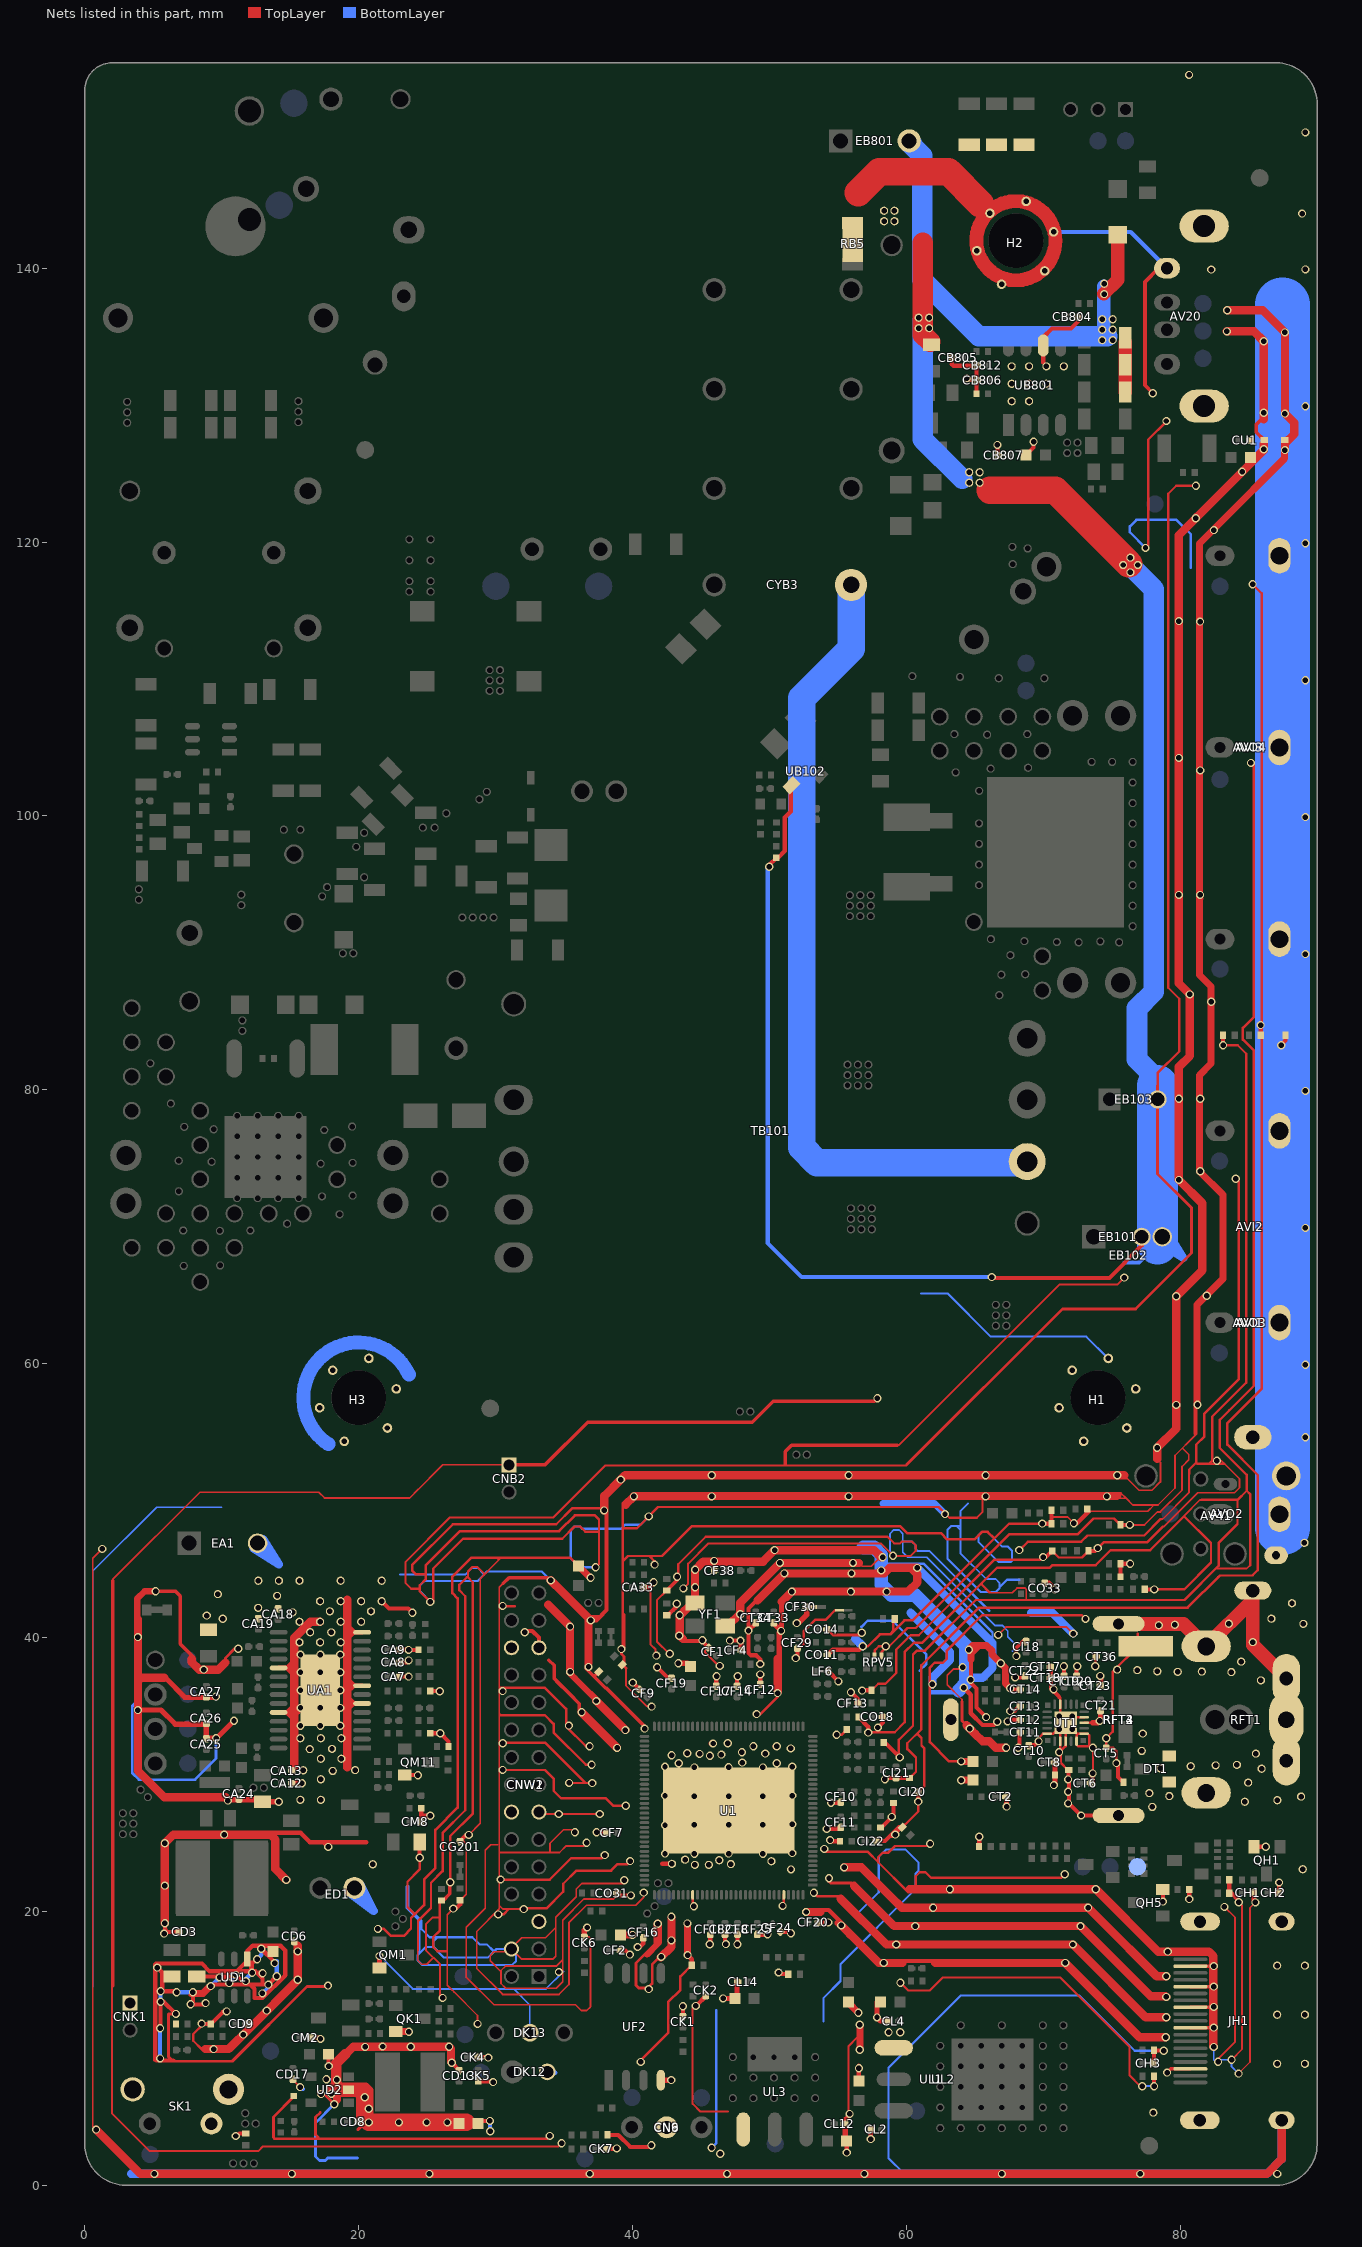
[diagram p0: the nets of this part, all layers, seen from the top]
# Altium PCB MISC116569.PcbDoc (part 9 of 15)
Units mm, origin at the board's own origin, x right, y up, seen from the top; angles counter-clockwise.
Board outline 90 x 155 mm, 2 copper layers (TopLayer, BottomLayer), stack 1.571 mm thick; 527 components, 277 nets, 2450 pads, 649 vias.

## Via types
v1: diameter 0.6, hole 0.4, TopLayer to BottomLayer, tented both sides, 649 vias

## Nets (pads, with @x,y where several pads share a name; then routed paths per layer and width w, separated by ;. In a path a pad name is that pad's centre, name@x,y a point inside that pad or via, vN(x,y) a via of type N, cw(c..) or ccw(c..) an arc to the next point about the centre after c; other vN are vias at no path point) (continued)
GND: (continued)
  TopLayer w0.3: v1(32.131,40.386) 32.233,40.488 32.677,40.488 33.164,40.001 CNW2.25@33.164,39.251 ; CF2.1@39.138,17.147 39.495,17.147 39.802,16.84 v1(39.816,16.84) ; v1(49.987,96.291) 49.854,96.291 RB134.1@50.503,96.94 v1@50.013,96.45 ; RB134.1@50.627,96.939 51.119,97.431 51.119,99.009 ; UB102.A@51.556,102.274 51.556,100.317 ; 63.32,132.992 CB805.2@63.32,133.477 ; v1(66.23,66.319) 66.285,66.265 74.837,66.265 77.187,68.615 EB101.2@77.187,69.266 ; 69.998,133.117 UB801.6@69.998,134.358 69.998,134.958 70.637,135.598 72.022,135.598 72.523,136.099 CB804.1@72.523,136.398 ; 51.119,99.009 51.119,99.88 51.556,100.317 ; 51.119,99.009 51.119,99.888 51.341,100.11 51.349,100.11 51.556,100.317
  TopLayer w0.305: 5.151,9.139 5.151,9.335 ; v1(5.299,15.89) 5.658,15.531 5.658,14.16 v1(5.532,14.16) 6.637,14.16 v1(6.701,14.097) ; v1@5.494,9.144 v1(5.494,9.258) ; v1(5.498,11.468) 5.536,11.506 v1(5.536,13.399) 5.763,13.399 v1(6.651,12.51) ; v1(5.791,18.377) 5.791,18.466 5.829,18.504 CD3.1@6.851,18.504 6.053,18.504 5.85,18.707 v1(5.85,19.139) ; 6.459,9.106 5.228,9.106 5.151,9.182 5.151,9.335 ; v1@7.742,13.881 8.664,13.881 9.438,14.655 12.987,14.655 ; CD1.2@8.174,15.241 10.717,15.241 UD1.1@11.855,16.38 ; v1(8.526,11.805) 8.558,11.773 RD6.1@9.204,11.773 10.118,12.687 v1(10.358,12.687) ; v1(8.822,13.297) 8.733,13.208 v1(7.729,13.208) 7.895,13.373 v1(7.895,14.097) 8.553,14.097 8.998,14.541 v1(9.203,14.541) ; v1(9.838,15.176) 10.128,15.176 v1(10.549,14.757) v1(10.549,14.757) ; v1(11.019,3.594) 11.07,3.543 11.291,3.765 DK1.A@11.562,3.765 ; v1(11.031,15.354) 11.476,14.91 v1(11.755,14.91) ; v1(11.572,11.003) 11.859,11.291 CD9.1@11.859,11.786 ; UD1.1@11.867,16.525 11.867,17.092 12.26,17.485 14.305,17.485 14.638,17.152 14.638,15.327 12.976,13.665 12.396,13.665 12.396,14.344 12.086,14.655 ; 12.149,16.243 12.149,15.587 v1(12.214,15.523) ; v1(12.581,16.497) 12.532,16.497 12.214,16.179 v1(12.214,15.523) ; v1(12.886,17.272) 13.864,16.294 v1(13.864,16.218) ; v1@12.917,13.951 v1(12.975,14.008) ; v1(12.979,15.481) 12.938,15.523 v1(12.214,15.523) ; v1@13.215,14.655 12.987,14.655 ; v1(13.295,12.756) 13.398,12.756 15.548,14.906 v1(15.548,15.009) ; v1(13.413,14.649) v1(14.022,15.259) ; CD6.1@15.299,17.749 15.553,17.495 v1(15.553,17.069) ; CM2.1@16.536,10.782 17.114,10.782 v1(17.214,10.682) ; CD16.1@17.808,9.563 17.808,8.704 v1(17.813,8.7) ; v1(20.445,6.426) 20.445,5.877 v1(20.745,5.577) ; v1(20.471,10.103) 20.133,10.103 20.107,10.13 v1(21.75,10.13) ; v1(20.745,4.585) v1(22.944,4.585) ; pad.VIA5@21.68,42.649 22.216,42.113 23.622,42.113 v1(23.927,41.808) ; CA7.1@22.964,37.145 23.64,37.145 v1(23.643,37.148) ; CA8.1@22.964,38.177 23.491,38.177 v1(23.643,38.329) ; CA9.1@22.964,39.107 23.626,39.107 v1(23.643,39.091) RA11.1@24.363,39.091 ; QM11.E@23.363,29.947 v1(24.328,29.947) ; v1(23.808,10.109) 24.76,10.109 ; v1(24.455,23.914) CM7.2@24.455,25.07 ; CM8.1@24.575,26.53 24.575,26.987 ; RM15.2@24.575,27.533 24.575,26.987 ; v1(24.963,4.585) 25.725,4.585 ; RA1.2@25.229,33.011 v1(25.958,33.011) 26.569,32.4 RM12.2@26.569,32.029 ; RA9.1@25.229,36.087 25.91,36.087 v1(25.916,36.081) ; v1(25.23,26.987) 24.575,26.987 ; v1(26.487,4.585) 27.851,4.585 ; v1(26.805,8.943) 26.811,8.943 CD13.1@27.338,8.416 ; v1(26.909,20.203) 26.91,20.201 27.116,20.201 27.414,20.499 RF13.2@27.414,20.812 ; CD15.1@27.345,4.49 CD15.1@27.413,4.559 ; CG201.2@27.414,25.144 27.85,25.58 v1(28.037,25.58) ; CD14.1@28.729,4.49 28.937,4.699 v1(29.591,4.699) ; CK5.2@28.735,7.566 29.7,7.566 v1@29.737,7.529 ; CK4.2@28.766,9.362 29.434,9.362 v1(29.472,9.324) ; v1(37.38,25.774) 37.395,25.758 CF7.1@38.057,25.758 ; CK7.2@38.156,2.657 38.819,2.657 v1(38.844,2.682) ; DK3.A@38.164,3.673 38.961,3.673 39.841,2.792 40.927,2.792 ; CO31.1@38.907,21.338 39.085,21.161 v1(39.886,21.161) ; v1(40.013,36.705) CF9.1@40.5,36.218 ; v1(40.372,17.397) 40.542,17.397 40.787,17.643 CF16.1@40.787,18.031 ; CA33.1@40.835,43.665 41.245,43.665 41.537,43.957 v1(41.537,44.033) ; v1(41.384,2.911) 41.266,2.792 40.927,2.792 ; v1@41.388,2.792 40.927,2.792 ; v1(41.796,37.833) 42.56,37.069 CF19.2@42.85,37.069 ; DI10.A@42.489,41.627 42.598,41.627 42.934,41.963 ; 43.124,42.154 42.934,41.963 ; v1(43.226,42.459) 43.188,42.459 43.162,42.484 43.162,42.192 42.934,41.963 ; v1@43.454,40.123 43.841,39.736 ; CK1.1@43.683,12.361 v1(43.683,13.071) ; 43.689,39.888 43.841,39.736 ; v1(44.023,16.808) 44.33,16.501 D102.A@44.33,16.081 ; v1(44.623,13.096) 44.597,13.122 44.667,13.122 CK2.2@45.347,13.801 ; v1@45.171,39.736 44.526,39.736 ; CF1.1@45.545,39.265 45.11,39.7 v1(45.11,39.802) 45.045,39.736 44.526,39.736 ; v1(45.639,17.605) 45.683,17.648 CF18.2@45.683,18.283 ; CF38.1@45.951,44.884 45.951,45.587 v1(45.956,45.593) ; CF17.1@46.114,36.491 46.114,37.147 v1(46.136,37.169) ; CF21.2@46.749,18.283 46.749,17.681 v1(46.824,17.605) ; v1(47.112,39.778) 47.113,39.779 v1(47.887,39.779) 47.887,39.141 CF4.1@47.96,39.068 v1@47.96,39.769 ; CF14.1@47.638,36.491 47.638,37.124 v1(47.683,37.169) ; v1(47.658,17.605) 47.666,17.613 CF8.1@47.666,18.283 ; CF12.1@49.335,36.622 v1(49.335,37.302) ; v1@49.335,38.292 v1(49.335,38.064) 49.335,38.398 49.031,38.701 48.647,38.701 48.471,38.877 48.471,40.5 CT34.2@49.002,41.031 48.474,40.503 v1(48.471,40.503) 48.471,42.118 49.452,43.099 ; 49.474,18.283 CF25.2@49.112,18.283 49.814,18.283 v1(49.863,18.332) ; v1(50.668,15.535) 50.782,15.42 D101.A@51.373,15.42 ; CF24.2@50.825,18.491 51.48,18.491 v1(51.567,18.404) ; v1(51.918,38.494) v1@52.04,38.616 ; v1@52.04,38.712 CF29.2@52.04,39.18 ; 53.157,19.953 53.31,20.105 54.334,20.105 55.878,18.56 ; CF20.1@53.612,19.192 v1(54.3,19.192) ; v1(54.178,26.022) 54.185,26.029 CF11.2@55.207,26.029 ; CO11.1@54.26,38.735 54.627,39.102 55.156,39.102 ; LF6.1@54.331,37.502 v1(55.042,36.792) v1@55.019,36.792 ; v1(54.432,25.209) 54.521,25.121 RV5.1@55.157,25.121 ; v1(54.496,27.927) 54.499,27.93 CF10.1@55.207,27.93 ; 54.772,39.102 55.156,39.102 ; v1(55.642,2.382) CL11.1@55.642,3.241 ; v1(55.956,36.005) 56.495,35.465 CF13.1@56.495,35.204 ; RO18.1@56.496,34.194 57.213,33.476 v1(57.213,33.058) ; v1(56.769,36.119) 56.794,36.144 DV7.A@57.462,36.144 ; v1(56.815,39.36) 56.557,39.102 55.156,39.102 ; CL2.1@57.393,4.079 57.393,3.374 v1(57.399,3.368) ; CI22.2@57.812,25.133 58.445,25.133 58.839,25.527 ; v1(57.925,33.426) 58.293,33.794 CO18.1@58.293,34.194 ; RF16.2@58.102,26.112 58.177,26.112 v1@58.928,26.863 ; RI18.1@58.346,32.334 58.43,32.334 v1@59.459,31.306 ; v1(58.433,29.642) 58.522,29.731 RV1.1@60.236,29.731 ; v1(58.928,26.899) v1@58.928,26.863 ; RV3.1@59.055,27.909 59.055,26.99 v1@58.928,26.863 ; v1(59.182,25.603) 59.106,25.527 58.839,25.527 ; 59.266,16.385 61.958,16.385 62.111,16.233 ; DV9.A@59.686,26.153 59.466,26.153 58.839,25.527 ; v1(60.871,28.016) CI20.2@60.871,28.727 ; 63.32,132.992 63.44,132.871 65.068,132.871 CB812.2@65.115,132.918 RB803.1@65.115,130.835 ; v1(64.186,36.335) 64.702,35.819 64.702,35.369 ; v1(64.414,131.953) 64.541,131.826 CB806.2@65.115,131.826 ; v1(64.691,36.909) 64.714,36.932 64.714,37.478 ; 64.702,35.608 64.702,35.369 ; 64.702,35.641 64.702,35.369 ; 64.714,38.832 64.714,37.478 ; 65.121,36.045 65.121,35.827 ; RH82.2@65.317,24.74 65.317,25.45 v1(65.316,25.451) ; v1(65.819,34.191) 65.121,34.889 65.121,35.827 ; v1(66.632,33.848) 66.399,33.615 65.556,33.615 64.702,34.47 64.702,35.369 ; CB807.1@66.652,126.34 v1(66.652,127.095) ; v1(67.394,33.873) 67.508,33.988 CT12.1@68.258,33.988 ; v1(67.581,34.631) 67.911,34.631 CT13.2@68.258,34.978 ; v1(67.584,36.299) 67.673,36.21 CT14.1@68.265,36.21 ; v1(67.94,37.086) 68.61,37.086 CT22.2@68.664,37.14 ; v1(68.169,31.956) 68.258,32.045 CT11.1@68.258,33.079 ; CB801.2@68.75,126.362 69.286,126.899 v1(69.286,127.33) ; CT10.1@68.943,32.139 69.368,32.139 v1(69.655,32.426) ; v1(69.931,48.317) 69.935,48.313 DI1.A@70.608,48.313 DA32.A@70.608,49.291 ; v1(69.98,45.876) 70.209,45.876 RO4.1@70.652,46.319 ; CO33.1@70.104,44.011 70.416,44.011 70.841,43.586 v1(70.841,43.523) ; CT17.2@70.558,37.848 70.558,36.69 ; v1(70.754,36.219) 70.738,36.219 70.558,36.399 70.558,36.69 ; 71.138,35.679 70.558,36.258 70.558,36.69 ; v1(71.505,37.897) 71.522,37.88 CT19.1@71.522,37.219 ; v1@71.852,29.784 LT4.1@71.852,30.324 ; v1@71.877,29.632 71.877,27.879 v1(72.756,27) RFT2.4@75.5,27 ; v1(72.233,48.339) 72.445,48.339 73.215,49.108 RA32.1@73.215,49.378 ; CT20.1@72.436,37.219 72.436,37.848 v1(72.487,37.899) ; DA33.A@73.305,46.319 73.776,46.319 v1(73.983,46.526) ; CT6.2@73.49,29.365 73.604,29.479 v1(73.604,30.076) ; v1(75.344,30.825) 75.458,30.711 75.458,29.816 LT1.1@75.859,29.416 ; RA31.1@75.642,44.44 DA31.A@75.642,45.379 v1(76.337,45.379) ; DI3.A@75.642,48.224 v1(76.322,48.224) ; DI2.A@77.413,43.513 v1(78.1,43.513) ; CH3.1@78.089,8.905 78.093,8.909 DH1.A@78.093,9.845 78.773,9.845 v1(78.799,9.82) ; v1(78.093,7.235) DH81.A@78.093,7.965 ; v1(78.735,20.716) QH5.E@78.735,21.58 ; v1(80.653,20.894) 80.659,20.9 RH59.1@80.659,21.605 ; 81.11,54.905 81.11,57.102 v1@81.212,57 ; v1(83.129,83.251) 83.13,83.252 DV4.A@83.13,83.988 ; DH3.A@83.586,22.304 DH2.A@83.586,21.338 83.743,21.338 84.277,20.804 v1(84.277,20.663) ; CH1.2@85.37,21.365 85.37,20.774 v1(85.491,20.653) ; QH1.E@85.377,24.717 v1(86.241,24.717) ; v1(85.872,84.724) 85.878,84.718 DV3.A@85.878,83.987 ; CH2.2@87.225,21.364 v1(87.225,22.106) ; v1(87.371,83.251) 87.371,83.289 87.682,83.6 DV5.A@87.682,83.987 DV5.A@87.682,83.79 ; 5.151,9.335 5.151,16.129 5.202,16.18 8.56,16.18 9.119,15.621 12.467,15.621 12.987,15.1 12.987,14.655 ; 43.841,39.736 44.526,39.736 ; 64.714,37.478 64.714,36.67 65.121,36.263 65.121,35.827
  TopLayer w0.33: 13.684,25.743 15.756,25.743 16.442,25.057 17.513,25.057 ; 15.273,33.985 14.729,34.529 UA1.24@14.154,34.529 ; 15.273,37.235 14.729,37.779 UA1.19@14.154,37.779 14.763,37.779 15.299,38.315 ; 15.299,35.065 14.763,34.529 UA1.24@14.154,34.529 ; 15.606,34.529 UA1.24@14.154,34.529 ; v1(17.78,24.701) 17.513,24.968 17.513,25.057 ; 19.109,34.644 19.645,35.179 UA1.6@20.254,35.179 19.678,35.179 19.135,35.723 ; 19.109,35.944 19.645,36.479 UA1.8@20.254,36.479 19.678,36.479 19.135,37.023 ; 19.109,39.844 19.645,40.379 UA1.14@20.254,40.379 19.678,40.379 19.135,40.923 ; 20.569,25.057 17.513,25.057 ; 42.177,23.47 pad.VIA5@42.883,23.47 ; CL1.1@56.54,7.598 v1(56.54,8.547) v1@56.54,8.738
  TopLayer w0.381: v1(3.883,34.701) 5.573,34.701 6.603,33.671 CA26.1@8.877,33.671 CA25.2@8.877,32.645 ; 5.872,37.067 7.325,35.614 CA27.2@8.878,35.614 9.505,35.614 v1(9.58,35.689) ; v1(9.588,32.639) 9.583,32.645 CA25.2@8.877,32.645 ; v1(10.452,28.092) 10.452,28.156 CA24.1@11.252,28.156 CA1.1@12.813,28.156 ; v1(10.897,33.922) 9.62,32.645 CA25.2@8.877,32.645 ; CA1.1@12.967,28.003 v1(14.16,28.003) ; CA12.1@15.177,29.357 15.857,29.357 v1(15.862,29.362) ; QM1.E@21.522,15.875 v1(21.522,16.739) ; CK6.1@36.482,18.144 36.482,18.623 v1(36.68,18.821) ; UF2.4@42.07,7.671 42.83,7.671 v1(42.832,7.673) ; v1(43.358,38.113) 44.001,38.113 CF3.1@44.221,37.892 ; v1(46.617,13.642) CL13.1@47.472,13.642 ; CL13.1@47.631,13.801 CL14.1@47.631,14.861 ; CT33.1@50.31,41.031 50.871,40.47 50.853,40.47 v1(50.846,40.477) ; 50.6,38.445 50.714,38.56 50.714,40.346 v1(50.846,40.477) ; 50.884,42.598 50.884,40.515 v1(50.846,40.477) ; v1(52.002,41.049) 52.129,41.049 52.719,41.639 CF30.2@52.719,42.23 ; CL11.1@55.532,3.35 CL12.1@55.532,4.486 55.532,4.778 55.85,5.095 v1(55.85,5.209) ; CL3.1@57.856,13.376 v1(57.856,12.258) 58.123,11.991 CL4.1@58.644,11.991 ; v1(67.318,27.648) 67.32,27.65 CT2.1@67.32,28.362 ; v1(70.777,29.223) 70.866,29.311 CT8.2@70.866,30.875 ; 73.596,33.779 73.987,33.779 v1(74.117,33.909) 74.168,33.909 74.181,33.922 CT21.1@74.181,34.61 ; v1(74.155,37.189) 74.206,37.139 CT23.2@74.206,36.487
  TopLayer w0.457: 3.883,41.331 3.834,41.38 3.834,42.848 4.369,43.383 v1(5.169,43.383) ; v1@35.365,37.456 35.796,37.024 ; v1(35.441,37.488) 35.441,37.38 35.796,37.024 ; 37.952,34.869 35.796,37.024 ; 41.062,16.85 41.842,17.63 41.842,17.738
  TopLayer w0.508: QK1.E@22.715,11.217 23.665,11.217 v1(23.668,11.214) ; CF15.1@36.22,45.21 CF15.1@36.063,45.21 v1@36.924,44.348 ; CD10.1@39.124,18.275 v1(40.005,18.275) ; 41.224,50.355 43.256,50.355 ; v1(44.013,19.116) 44.013,16.818 v1(44.023,16.808) ; v1(45.779,2.743) v1@45.791,2.756 ; v1@45.815,32.259 v1(45.885,32.259) ; YF1.2@46.896,40.833 YF1.2@46.949,40.833 ; v1@46.941,32.259 v1(46.956,32.274) ; UL3.1@48.089,3.612 UL3.1@48.089,4.072 ; v1@50.472,32.056 v1(50.533,32.056) ; CF5.1@55.761,13.393 55.761,13.325 v1(56.497,12.588) ; v1(56.599,9.896) 56.599,10.798 v1(56.599,11.725) ; v1(64.016,29.578) 64.018,29.581 CT1.1@64.876,29.581 ; v1(64.016,30.95) 64.018,30.952 CT52.1@64.876,30.952 ; v1(64.567,39.103) 64.567,39.167 64.829,39.429 65.854,39.429 ; 64.714,38.405 64.714,38.832 65.311,39.429 ; 65.583,39.429 65.854,39.429 ; v1(65.784,50.305) 65.834,50.355 66.332,50.355 ; v1(66.891,38.113) 66.891,38.138 66.523,38.506 ; 67.254,37.48 67.254,37.097 ; v1(67.584,36.299) 67.254,36.629 67.254,37.097 ; v1@74.638,50.288 73.952,50.288 ; v1@74.651,50.288 v1(74.651,50.305) ; 75.391,50.288 73.952,50.288 ; 75.458,50.355 66.332,50.355 ; v1@81.212,57 81.212,58.08 ; v1(81.262,57) 81.212,57.051 81.212,58.08 ; v1@81.448,93.959 81.402,94.005 v1@81.402,94.412 ; v1(81.458,74.054) 81.402,74.109 81.402,74.79 ; v1(81.458,79.35) 81.402,79.294 81.402,78.892 ; v1(81.458,103.327) 81.453,103.327 81.402,103.378 81.402,104.191 ; v1(81.94,64.96) 81.872,64.96 83.109,66.197 83.109,72.334 81.402,74.04 81.402,74.79 ; 82.248,87.493 v1@82.248,86.436 ; v1(82.461,120.879) 82.461,120.949 83.023,121.51 ; 82.99,66.078 81.212,64.3 81.212,58.08 ; DU1.A@87.6,127.317 87.6,126.136 ; v1(87.651,126.721) 87.612,126.721 87.6,126.733 87.6,126.136 ; 43.256,50.355 66.332,50.355 ; 43.256,50.355 43.332,50.279 72.602,50.279 72.61,50.288 73.952,50.288 ; 65.854,39.429 66.238,39.045 66.238,38.791 66.523,38.506 ; 66.523,38.506 67.254,37.775 67.254,37.097 ; 81.402,74.79 81.402,78.892 ; 81.402,78.892 81.402,81.062 82.248,81.908 v1@82.248,86.436 ; v1@81.402,94.412 81.402,88.389 82.248,87.543 v1@82.248,86.436 ; v1@81.402,94.412 81.402,104.191 ; 81.402,104.191 81.402,119.89 83.023,121.51 ; 83.023,121.51 87.6,126.087 87.6,126.136
  TopLayer w0.584: v1(59.266,17.579) 59.647,17.579 ; v1(61.954,20.268) 61.958,20.272 63.373,20.272 ; 63.919,21.618 v1(63.178,21.618) 64.359,21.618
  TopLayer w0.61: v1(0.826,4.064) 4.064,0.826 6.79,0.826 ; v1(3.883,34.701) 3.883,35.45 ; v1(3.883,40.03) 3.883,40.45 ; 3.883,41.331 3.883,40.45 ; 4.582,0.826 6.79,0.826 ; 5.795,37.067 4.128,37.067 3.883,36.822 ; v1(5.85,19.139) pad.VIA5@5.85,24.977 6.479,25.606 13.547,25.606 13.914,25.238 13.914,24.879 ; 7.805,38.451 7.805,38.207 8.357,37.655 ; 8.109,37.904 8.357,37.655 ; 8.796,9.944 9.939,9.944 ; v1(9.406,9.944) 9.939,9.944 ; 10.274,38.173 9.757,37.655 8.357,37.655 ; v1@10.452,28.156 10.283,28.325 5.812,28.325 3.883,30.255 3.883,35.45 ; 11.859,11.29 12.061,11.493 ; 13.914,23.525 13.914,24.879 ; v1(14.714,22.296) 13.914,23.096 13.914,24.879 ; 15.299,30.594 15.299,38.43 ; 15.299,38.722 15.299,38.43 ; 15.553,17.495 15.553,14.984 12.061,11.493 ; pad.VIA5@17.18,41.149 16.473,41.149 15.299,39.975 15.299,38.43 ; 18.423,6.238 18.423,8.931 19.601,10.109 v1(26.609,10.109) ; 19.172,30.505 19.172,42.748 ; 24.76,10.109 v1(26.609,10.109) ; v1@26.801,8.94 26.741,9 26.741,9.977 v1(26.609,10.109) ; CNW2.25@33.164,39.071 CNW2.25@33.164,39.251 ; 33.849,42.386 v1(35.441,40.794) v1(35.441,37.488) ; v1(34.03,44.169) 34.746,43.453 ; v1@34.168,44.031 34.746,43.453 ; v1(36.279,34.542) v1@38.872,31.949 ; v1@36.787,38.128 36.787,40.655 36.787,41.412 34.746,43.453 ; v1(37.363,35.362) v1(39.482,33.243) ; v1(37.924,49.277) 37.947,49.301 37.947,50.343 v1(39.141,51.537) 39.459,51.854 70.269,51.854 ; 39.497,49.701 v1(40.101,50.305) v1(45.783,50.305) ; 41.842,17.738 v1(41.842,19.091) ; v1@42.061,16.627 42.845,17.412 v1@42.845,19.545 ; v1(43.417,40.129) 43.454,40.167 43.454,40.678 ; v1(43.442,41.618) 43.465,41.618 43.79,41.943 ; 43.689,39.888 43.454,40.123 43.454,40.678 ; YF1.2@46.82,40.833 46.945,40.833 47.876,41.764 47.876,42.154 ; v1(47.874,41.697) 47.876,41.698 47.876,42.154 ; 49.13,42.713 v1(51.095,44.677) ; v1@50.6,36.043 50.6,37.379 ; 50.6,37.899 50.6,37.379 ; 50.6,38.445 50.6,37.379 ; 50.884,42.598 v1(51.642,43.356) v1(55.956,43.356) 57.201,43.356 ; 51.468,44.677 v1(51.095,44.677) ; v1(52.675,19.953) 53.157,19.953 53.729,19.953 ; v1@55.07,19.153 56.177,18.046 ; 55.21,20.918 58.548,17.579 59.647,17.579 v1(72.16,17.579) ; v1(55.454,23.212) 56.723,23.212 58.874,21.061 ; 55.828,18.396 56.177,18.046 ; 56.174,21.858 59.106,18.925 v1(60.65,18.925) v1(72.717,18.925) 77.837,13.806 78.927,13.806 v1(78.983,13.75) ; 56.54,45.443 v1(50.77,45.443) 47.876,42.549 47.876,42.154 ; v1(58.161,44.897) 57.941,44.677 56.993,44.677 ; v1(58.263,45.862) 58.166,45.862 57.645,46.383 v1(50.38,46.383) 49.538,45.541 45.165,45.541 v1(44.569,44.945) v1(44.569,43.665) YF1.4@44.569,42.533 44.38,42.533 43.79,41.943 ; v1(58.352,16.233) 59.317,16.233 ; v1(58.56,43.356) 57.201,43.356 ; 59.33,20.605 58.874,21.061 ; 59.714,16.233 59.317,16.233 ; 60.121,43.356 57.201,43.356 ; 60.168,43.403 60.798,44.033 60.798,44.618 60.333,45.083 59.698,45.083 ; 60.234,21.618 62.708,21.618 63.919,21.618 64.359,21.618 v1(73.833,21.618) 78.389,17.062 v1(79.086,17.062) 80.78,17.062 ; v1(60.798,45.083) 59.698,45.083 ; 62.111,16.233 v1(71.602,16.233) 77.029,10.806 v1(78.939,10.806) ; 64.395,33.592 65.025,32.962 ; v1(64.637,33.349) 65.025,32.962 ; v1(67.28,31.956) 66.518,31.956 66.048,32.426 65.561,32.426 65.025,32.962 ; 71.522,51.854 70.269,51.854 ; v1(75.4,51.854) 74.778,51.854 ; 75.921,51.854 74.778,51.854 ; 78.313,53.038 v1(78.313,53.859) ; 78.313,53.35 v1(78.313,53.859) ; v1@78.982,12.263 78.977,12.268 77.471,12.268 72.394,17.345 ; v1(78.983,15.262) 78.285,15.262 74.165,19.382 ; v1(79.904,79.35) 79.904,79.68 ; 80.31,17.062 80.78,17.062 ; v1(81.136,121.743) 81.519,122.126 ; v1(82.449,10.101) 82.423,10.127 82.423,16.733 82.094,17.062 80.78,17.062 ; v1(83.409,135.384) 85.383,135.384 v1(86.101,134.666) v1(86.101,129.451) 86.101,128.958 ; v1(83.434,136.934) 86.025,136.934 v1(87.651,135.308) v1(87.651,129.387) 88.332,128.705 88.332,127.897 87.651,127.216 v1(87.651,126.721) ; v1(84.522,125.129) 84.757,125.364 ; 86.101,127.165 86.101,126.708 84.757,125.364 ; JH1.21@87.409,4.75 87.409,1.907 86.327,0.826 6.79,0.826 ; 3.883,35.45 3.883,36.822 ; 3.883,36.822 3.883,40.45 ; 9.939,9.944 10.512,9.944 12.061,11.493 ; 43.454,40.678 43.454,41.608 43.79,41.943 ; v1(51.095,44.677) v1(55.994,44.677) 56.993,44.677 ; 56.177,18.046 57.99,16.233 59.317,16.233 ; 56.993,44.677 58.377,44.677 58.783,45.083 59.698,45.083 ; 58.874,21.061 59.663,20.272 63.373,20.272 v1(73.275,20.272) ; 70.269,51.854 74.778,51.854 ; v1(72.16,17.579) 72.394,17.345 ; v1(72.16,17.579) 72.394,17.345 ; v1(73.275,20.272) 74.165,19.382 ; v1(73.275,20.272) 74.165,19.382 ; v1(78.313,53.859) 79.713,55.259 v1(79.713,56.985) v1(79.713,64.92) 81.61,66.818 81.61,71.713 v1(79.904,73.42) 79.904,79.68 ; 79.904,79.68 79.904,81.683 80.704,82.483 v1(80.704,86.968) 79.904,87.768 v1(79.904,94.234) 79.904,120.51 81.519,122.126 ; 81.519,122.126 84.757,125.364
  TopLayer w0.762: 19.029,9.569 18.366,8.906 18.366,7.414 18.663,7.117 20.478,7.117 ; UD2.2@19.35,7.117 20.478,7.117 ; 20.699,5.997 20.699,6.896 20.478,7.117
  TopLayer w1: pad.VIA5@74.417,138.133 75.433,139.149 75.433,141.783 ; 75.433,141.097 75.433,141.783 ; DB804.K@75.433,142.445 75.433,141.783 ; RB820.1@75.993,130.963 RB818.1@75.993,134.592
  TopLayer w1.016: v1@18.118,6.96 19.937,6.96 20.445,6.452 v1(20.445,6.426) ; RFT2.3@75.5,41 80.25,41 RFT1.4@81.9,39.35 85.3,42.75 85.3,39.45 RFT3.6@87.75,37 ; 70.888,142.004 ccw(c68,142.004) 70.888,142.004
  TopLayer w1.27: v1(20.445,6.426) 20.445,4.885 v1(20.745,4.585) 27.851,4.585
  TopLayer w1.5: 61.209,135.496 61.209,137.274 ; 61.209,141.872 61.209,137.274 ; CB811.1@61.735,134.633 61.209,135.158 61.209,137.274
  TopLayer w2: 56.49,145.504 58.026,147.041 63.081,147.041 65.405,144.717 ; 66.111,123.774 70.861,123.774 76.233,118.402
  BottomLayer w0.127: 0.584,14.453 0.584,44.856 5.245,49.517 9.994,49.517 ; v1@21.528,16.745 23.938,14.336 28.85,14.336 ; 25.962,14.336 28.85,14.336 ; DK13.2@32.503,11.129 32.503,13.164 31.331,14.336 29.065,14.336 ; v1(34.628,15.57) v1@34.683,15.57 ; 34.971,15.621 33.686,14.336 29.065,14.336 ; v1@39.454,22.322 v1@39.454,22.329 ; v1(39.886,21.161) v1@40.054,21.161 ; v1(59.025,45.964) 58.807,46.181 58.807,47.584 59.08,47.856 59.465,47.856 59.737,47.584 59.737,46.232 60.107,45.862 61.485,45.862 66.466,40.881 66.992,40.881 67.399,40.475 67.399,40.052 67.846,39.604 67.846,39.106 67.754,39.014 ; 63.675,48.131 63.947,47.858 ; 64.514,49.799 63.947,49.233 63.947,47.858 ; 66.821,43.968 66.52,44.27 65.822,44.27 63.947,46.144 63.947,47.858 ; v1(82.449,10.101) 82.449,9.141 82.58,9.01 v1(82.766,9.01) 82.928,9.172 83.739,9.172 v1(83.752,9.159) 83.752,8.664 v1(84.26,8.156) ; 28.85,14.336 29.065,14.336
  BottomLayer w0.152: 23.023,44.613 26.289,44.613 ; 23.622,21.857 23.622,20.287 24.598,19.312 24.598,18.686 25.176,18.108 25.758,18.108 ; 24.589,16.129 24.309,16.409 24.309,16.805 24.9,17.396 25.463,17.396 ; 24.628,16.09 31.224,16.09 31.491,16.356 31.491,16.924 CNW2.4@31.164,17.251 30.068,17.251 29.845,17.028 ; v1@25.235,42.52 25.235,42.608 24.478,43.366 24.478,43.81 24.798,44.13 28.687,44.13 ; 26.086,44.13 28.687,44.13 ; 26.086,44.613 26.289,44.613 ; v1(34.03,44.169) 33.38,44.818 29.375,44.818 29.138,44.581 ; v1@41.681,38.684 v1(41.745,38.684) ; v1@42.624,38.913 v1(42.726,38.811) ; v1(43.251,44.44) v1@43.4,44.291 ; v1(43.721,43.588) v1@43.798,43.665 ; v1(50.96,20.399) v1@51.036,20.475 ; 53.962,11.951 53.962,13.686 55.186,14.91 55.186,16.146 60.663,21.622 60.663,22.728 60.879,22.944 60.879,23.576 59.949,24.506 58.511,24.506 57.986,23.982 57.986,21.398 56.445,19.856 ; v1@59.012,45.964 v1(59.025,45.964) ; 59.737,47.005 59.745,47.013 60.404,47.013 60.684,46.733 60.684,46.451 60.777,46.357 ; 59.84,0.826 58.694,1.971 58.694,8.572 63.978,13.856 72.639,13.856 76.675,9.82 v1(78.799,9.82) ; 60.803,46.332 61.68,46.332 66.074,41.938 ; 61.074,65.126 63.023,65.126 66.173,61.976 73.151,61.976 H1.3@74.75,60.377 ; 62.995,47.78 62.995,47.526 ; 63.947,48.085 63.889,48.143 63.284,48.143 62.995,47.854 62.995,47.526 ; 66.805,43.669 67.352,44.216 68.256,44.216 ; 66.805,43.952 66.805,43.607 66.525,43.327 65.439,43.327 62.995,45.771 62.995,47.526 ; v1(71.564,22.708) v1@71.653,22.708 ; v1(77.22,7.235) v1(78.093,7.235) ; 25.463,17.396 26.237,16.623 29.44,16.623 29.845,17.028 ; 25.463,17.396 25.463,17.813 25.758,18.108 ; 25.758,18.108 28.308,18.108 28.829,17.587 29.365,17.587 29.845,17.107 29.845,17.028 ; 26.289,44.613 27.818,44.613 28.291,45.086 28.687,45.086 29.138,44.635 29.138,44.581 ; 28.687,44.13 29.138,44.581 ; 65.256,46.987 65.256,47.45 65.523,47.717 65.919,47.717 67.002,46.633 67.426,46.633 67.706,46.354 67.706,45.596 67.614,45.504 66.739,45.504 65.256,46.987
  BottomLayer w0.178: v1@25.235,42.52 v1(25.235,42.596) ; v1@30.513,30.302 v1(30.513,30.328) ; v1(35.36,33.564) v1@35.36,33.696 ; v1(37.016,30.711) v1@37.054,30.673 ; v1@37.016,32.032 v1@37.041,32.057 ; v1(37.308,45.126) 36.147,45.126 35.484,45.789 35.484,47.818 35.771,48.105 36.177,48.105 36.355,47.927 39.148,47.927 39.453,48.232 40.574,48.232 v1(41.186,48.844) ; v1@38.757,32.057 v1(38.877,31.937) ; v1(45.779,2.743) 46.127,3.091 46.127,12.763 ; v1@54,24.457 v1(54,24.562) ; 56.715,40.78 57.163,41.227 58.991,41.227 61.464,38.754 61.464,38.061 60.98,37.577 ; v1@56.815,40.3 56.866,40.35 v1@56.866,40.447 ; v1@58.166,45.583 58.369,45.38 61.285,45.38 66.289,40.376 66.289,39.596 ; v1(73.8,37.906) v1@73.829,37.935 ; v1@74.595,32.591 v1(74.595,32.641) ; v1(77.465,119.57) 76.322,120.713 76.322,121.145 76.8,121.623 79.731,121.623 80.767,120.587 80.767,118.123 ; 87.11,73.726 87.25,73.866
  BottomLayer w0.203: 4.034,35.547 3.462,34.976 3.462,30.117 3.962,29.616 8.052,29.616 9.588,31.153 v1(9.588,32.639) ; v1(17.254,6.655) 17.991,6.655 v1(18.016,6.68) ; v1(17.648,7.734) 18.372,7.734 v1(18.41,7.696) ; v1(18.22,5.918) 16.858,4.556 16.858,2.091 17.14,1.808 17.569,1.808 17.742,1.981 19.926,1.981 ; v1(33.955,3.597) v1@34.024,3.528 ; v1(39.187,39.157) 39.213,39.131 v1@39.238,39.131 ; v1(56.749,40.341) v1@56.758,40.35